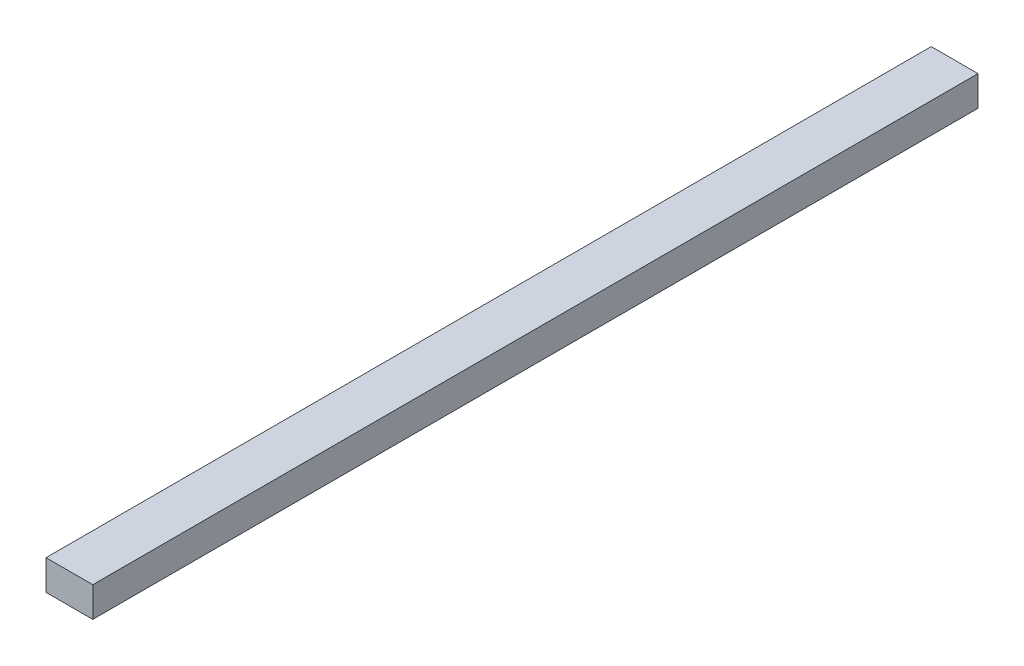
from build123d import *

# Parameters (mm, degrees)
SKETCH1_W           = 14
SKETCH1_H           = 265
BOSS_EXTRUDE1_DEPTH = 9


with BuildPart() as part:
    # Sketch1 → Boss-Extrude1 (new body)
    with BuildSketch(Plane(origin=(0, 164.943963655, 0), x_dir=(1, 0, 0), z_dir=(0, 1, 0))):
        with Locations((521.230642584, 793.192981355)):
            Rectangle(SKETCH1_W, SKETCH1_H)
    extrude(amount=-BOSS_EXTRUDE1_DEPTH)


solid = part.part
